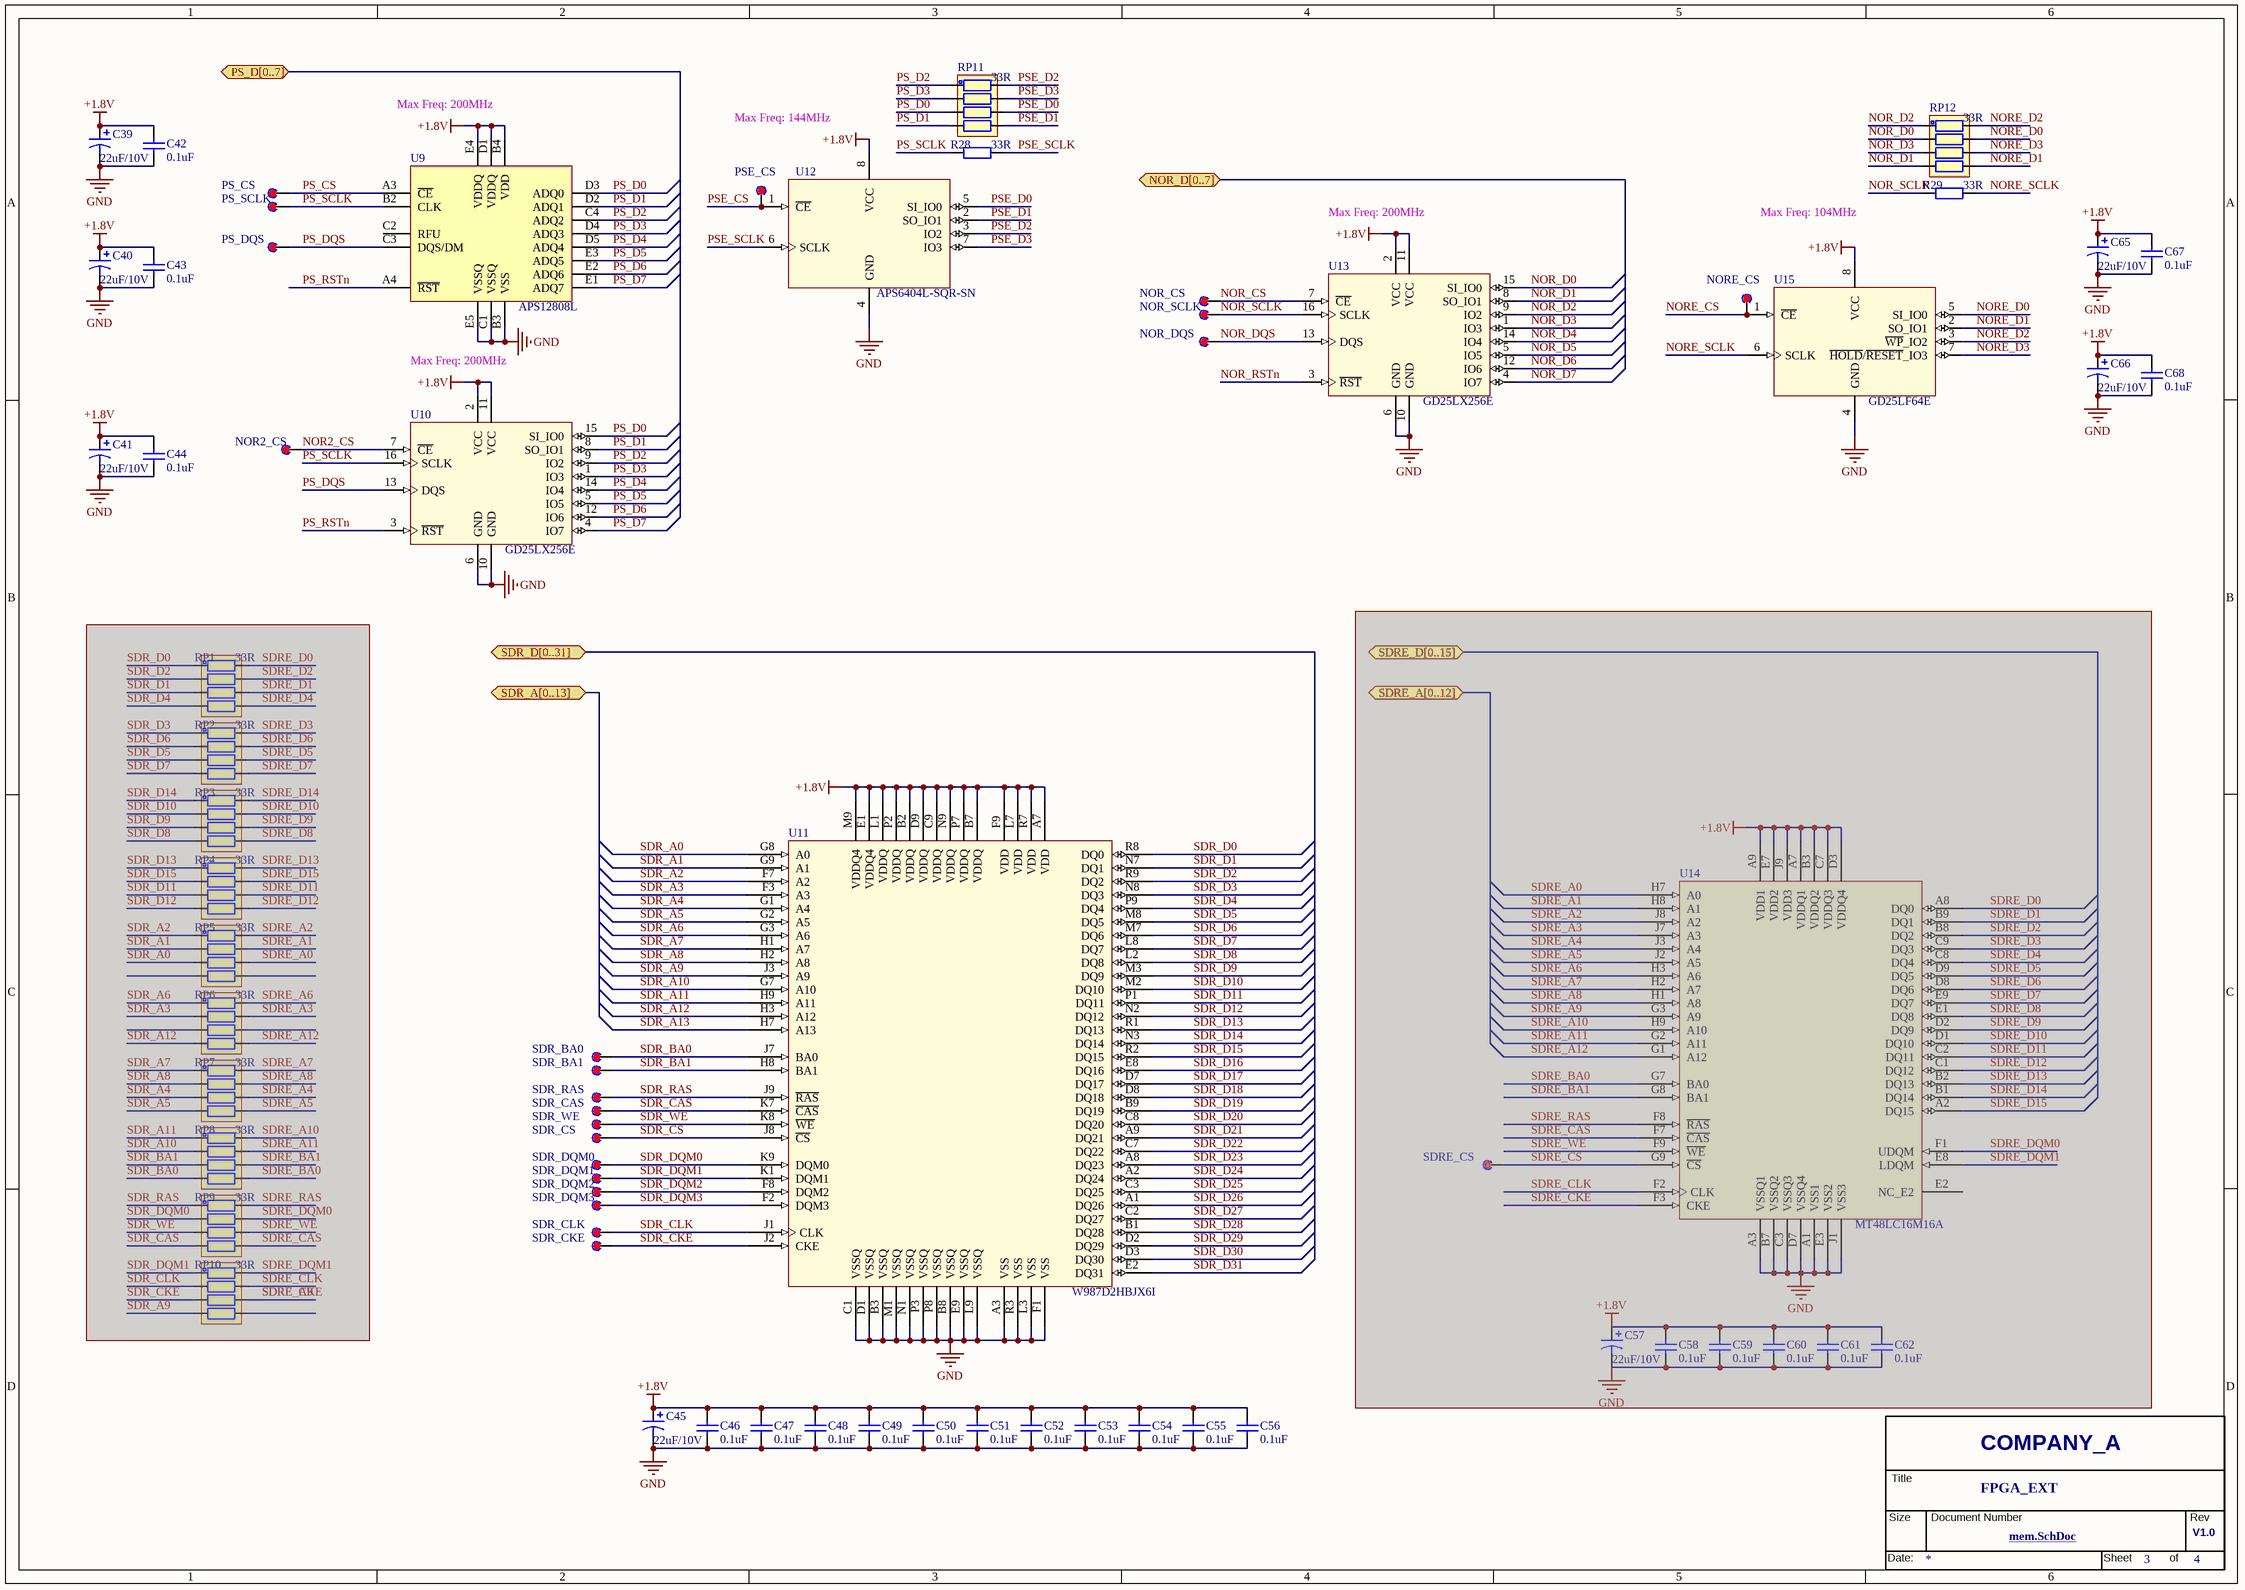
[diagram p0: MISC105414-7.SchDoc]
# Altium project MISC105414-4.PrjPcb (part 2 of 3)
## Sheet MISC105414-7.SchDoc
size 420 x 297 mm; DocumentNumber: MISC105414; SheetNumber: 2; SheetTotal: 4

### Parts
(Parts that share a designator on the sheet are numbered #1, #2 ... from top to bottom, then left to right.)
*?#3  Page Count: 4  Page Number: 3  OrgName: COMPANY_A  Title: FPGA_EXT  RevCode: V1.0  Doc: mem.SchDoc  (hidden comment: TitleBlock_YHSCH)  (graphical)
C39  22uF/10V  [0603C_N]
C40  22uF/10V  [0603C_N]
C41  22uF/10V  [0603C_N]
C42  0.1uF  [0603C_N]
C43  0.1uF  [0603C_N]
C44  0.1uF  [0603C_N]
C45  22uF/10V  [0603C_N]
C46  0.1uF  [0603C_N]
C47  0.1uF  [0603C_N]
C48  0.1uF  [0603C_N]
C49  0.1uF  [0603C_N]
C50  0.1uF  [0603C_N]
C51  0.1uF  [0603C_N]
C52  0.1uF  [0603C_N]
C53  0.1uF  [0603C_N]
C54  0.1uF  [0603C_N]
C55  0.1uF  [0603C_N]
C56  0.1uF  [0603C_N]
C57  22uF/10V  [0603C_N]  (masked out: inside a compile mask, not in the netlist)
C58  0.1uF  [0603C_N]  (masked out: inside a compile mask, not in the netlist)
C59  0.1uF  [0603C_N]  (masked out: inside a compile mask, not in the netlist)
C60  0.1uF  [0603C_N]  (masked out: inside a compile mask, not in the netlist)
C61  0.1uF  [0603C_N]  (masked out: inside a compile mask, not in the netlist)
C62  0.1uF  [0603C_N]  (masked out: inside a compile mask, not in the netlist)
C65  22uF/10V  [0603C_N]
C66  22uF/10V  [0603C_N]
C67  0.1uF  [0603C_N]
C68  0.1uF  [0603C_N]
R28  33R  [0603R_N]
R29  33R  [0603R_N]
RP1  33R  [0402RP-4P]  (masked out: inside a compile mask, not in the netlist)
RP2  33R  [0402RP-4P]  (masked out: inside a compile mask, not in the netlist)
RP3  33R  [0402RP-4P]  (masked out: inside a compile mask, not in the netlist)
RP4  33R  [0402RP-4P]  (masked out: inside a compile mask, not in the netlist)
RP5  33R  [0402RP-4P]  (masked out: inside a compile mask, not in the netlist)
RP6  33R  [0402RP-4P]  (masked out: inside a compile mask, not in the netlist)
RP7  33R  [0402RP-4P]  (masked out: inside a compile mask, not in the netlist)
RP8  33R  [0402RP-4P]  (masked out: inside a compile mask, not in the netlist)
RP9  33R  [0402RP-4P]  (masked out: inside a compile mask, not in the netlist)
RP10  33R  [0402RP-4P]  (masked out: inside a compile mask, not in the netlist)
RP11  33R  [0402RP-4P]
RP12  33R  [0402RP-4P]
TP18  PS_CS  [FZ_TP-SMD-Mini]
TP19  PS_SCLK  [FZ_TP-SMD-Mini]
TP20  PS_DQS  [FZ_TP-SMD-Mini]
TP21  NOR2_CS  [FZ_TP-SMD-Mini]
TP22  SDR_BA0  [FZ_TP-SMD-Mini]
TP23  SDR_BA1  [FZ_TP-SMD-Mini]
TP24  SDR_RAS  [FZ_TP-SMD-Mini]
TP25  SDR_CAS  [FZ_TP-SMD-Mini]
TP26  SDR_WE  [FZ_TP-SMD-Mini]
TP27  SDR_CS  [FZ_TP-SMD-Mini]
TP28  SDR_DQM0  [FZ_TP-SMD-Mini]
TP29  SDR_DQM1  [FZ_TP-SMD-Mini]
TP30  SDR_DQM2  [FZ_TP-SMD-Mini]
TP31  SDR_DQM3  [FZ_TP-SMD-Mini]
TP32  SDR_CLK  [FZ_TP-SMD-Mini]
TP33  SDR_CKE  [FZ_TP-SMD-Mini]
TP34  PSE_CS  [FZ_TP-SMD-Mini]
TP35  NOR_CS  [FZ_TP-SMD-Mini]
TP36  NOR_SCLK  [FZ_TP-SMD-Mini]
TP37  NOR_DQS  [FZ_TP-SMD-Mini]
TP38  SDRE_CS  [FZ_TP-SMD-Mini]  (masked out: inside a compile mask, not in the netlist)
TP39  NORE_CS  [FZ_TP-SMD-Mini]
U9  APS12808L  [PBGA24 6X8]
U10  GD25LX256E  [SOIC16]
U11  W987D2HBJX6I  [VFBGA90_8X13]
U12  APS6404L-SQR-SN  [SOP8]
U13  GD25LX256E  [SOIC16]
U14  MT48LC16M16A  [VFBGA54_8X9]  (masked out: inside a compile mask, not in the netlist)
U15  GD25LF64E  [SOIC8]

### Ports
NOR_D[0..7], PS_D[0..7], SDR_A[0..13], SDR_D[0..31], SDRE_A[0..12], SDRE_D[0..15]

### Nets
+1.8V: C39.1 C40.1 C41.1 C42.2 C43.2 C44.2 C45.1 C46.2 C47.2 C48.2 C49.2 C50.2 C51.2 C52.2 C53.2 C54.2 C55.2 C56.2 C65.1 C66.1 C67.2 C68.2 U9.B4(VDD) U9.D1(VDDQ) U9.E4(VDDQ) U10.2(VCC) U10.11(VCC) U11.A7(VDD) U11.B2(VDDQ) U11.B7(VDDQ) U11.C9(VDDQ) U11.D9(VDDQ) U11.E1(VDDQ4) U11.F9(VDD) U11.L1(VDDQ) U11.L7(VDD) U11.M9(VDDQ4) U11.N9(VDDQ) U11.P2(VDDQ) U11.P7(VDDQ) U11.R7(VDD) U12.8(VCC) U13.2(VCC) U13.11(VCC) U15.8(VCC)
GND: C39.2 C40.2 C41.2 C42.1 C43.1 C44.1 C45.2 C46.1 C47.1 C48.1 C49.1 C50.1 C51.1 C52.1 C53.1 C54.1 C55.1 C56.1 C65.2 C66.2 C67.1 C68.1 U9.B3(VSS) U9.C1(VSSQ) U9.E5(VSSQ) U10.6(GND) U10.10(GND) U11.A3(VSS) U11.B3(VSSQ) U11.B8(VSSQ) U11.C1(VSSQ) U11.D1(VSSQ) U11.E9(VSSQ) U11.F1(VSS) U11.L3(VSS) U11.L9(VSSQ) U11.M1(VSSQ) U11.N1(VSSQ) U11.P3(VSSQ) U11.P8(VSSQ) U11.R3(VSS) U12.4(GND) U13.6(GND) U13.10(GND) U15.4(GND)
NOR2_CS: TP21.1 U10.7(~{CE})
NOR_CS: TP35.1 U13.7(~{CE})
NOR_D0: RP12.2 U13.15(SI_IO0)
NOR_D1: RP12.4 U13.8(SO_IO1)
NOR_D2: RP12.1 U13.9(IO2)
NOR_D3: RP12.3 U13.1(IO3)
NOR_D4: U13.14(IO4)
NOR_D5: U13.5(IO5)
NOR_D6: U13.12(IO6)
NOR_D7: U13.4(IO7)
NOR_DQS: TP37.1 U13.13(DQS)
NOR_RSTn: U13.3(~{RST})
NOR_SCLK: R29.2 TP36.1 U13.16(SCLK)
NORE_CS: TP39.1 U15.1(~{CE})
NORE_D0: RP12.7 U15.5(SI_IO0)
NORE_D1: RP12.5 U15.2(SO_IO1)
NORE_D2: RP12.8 U15.3(~{WP}_IO2)
NORE_D3: RP12.6 U15.7(~{HOLD}/~{RESET}_IO3)
NORE_SCLK: R29.1 U15.6(SCLK)
PS_CS: TP18.1 U9.A3(~{CE})
PS_D0: RP11.3 U9.D3(ADQ0) U10.15(SI_IO0)
PS_D1: RP11.4 U9.D2(ADQ1) U10.8(SO_IO1)
PS_D2: RP11.1 U9.C4(ADQ2) U10.9(IO2)
PS_D3: RP11.2 U9.D4(ADQ3) U10.1(IO3)
PS_D4: U9.D5(ADQ4) U10.14(IO4)
PS_D5: U9.E3(ADQ5) U10.5(IO5)
PS_D6: U9.E2(ADQ6) U10.12(IO6)
PS_D7: U9.E1(ADQ7) U10.4(IO7)
PS_DQS: TP20.1 U9.C3(DQS/DM) U10.13(DQS)
PS_RSTn: U9.A4(~{RST}) U10.3(~{RST})
PS_SCLK: R28.2 TP19.1 U9.B2(CLK) U10.16(SCLK)
PSE_CS: TP34.1 U12.1(~{CE})
PSE_D0: RP11.6 U12.5(SI_IO0)
PSE_D1: RP11.5 U12.2(SO_IO1)
PSE_D2: RP11.8 U12.3(IO2)
PSE_D3: RP11.7 U12.7(IO3)
PSE_SCLK: R28.1 U12.6(SCLK)
SDR_A0: U11.G8(A0)
SDR_A1: U11.G9(A1)
SDR_A2: U11.F7(A2)
SDR_A3: U11.F3(A3)
SDR_A4: U11.G1(A4)
SDR_A5: U11.G2(A5)
SDR_A6: U11.G3(A6)
SDR_A7: U11.H1(A7)
SDR_A8: U11.H2(A8)
SDR_A9: U11.J3(A9)
SDR_A10: U11.G7(A10)
SDR_A11: U11.H9(A11)
SDR_A12: U11.H3(A12)
SDR_A13: U11.H7(A13)
SDR_BA0: TP22.1 U11.J7(BA0)
SDR_BA1: TP23.1 U11.H8(BA1)
SDR_CAS: TP25.1 U11.K7(~{CAS})
SDR_CKE: TP33.1 U11.J2(CKE)
SDR_CLK: TP32.1 U11.J1(CLK)
SDR_CS: TP27.1 U11.J8(~{CS})
SDR_D0: U11.R8(DQ0)
SDR_D1: U11.N7(DQ1)
SDR_D2: U11.R9(DQ2)
SDR_D3: U11.N8(DQ3)
SDR_D4: U11.P9(DQ4)
SDR_D5: U11.M8(DQ5)
SDR_D6: U11.M7(DQ6)
SDR_D7: U11.L8(DQ7)
SDR_D8: U11.L2(DQ8)
SDR_D9: U11.M3(DQ9)
SDR_D10: U11.M2(DQ10)
SDR_D11: U11.P1(DQ11)
SDR_D12: U11.N2(DQ12)
SDR_D13: U11.R1(DQ13)
SDR_D14: U11.N3(DQ14)
SDR_D15: U11.R2(DQ15)
SDR_D16: U11.E8(DQ16)
SDR_D17: U11.D7(DQ17)
SDR_D18: U11.D8(DQ18)
SDR_D19: U11.B9(DQ19)
SDR_D20: U11.C8(DQ20)
SDR_D21: U11.A9(DQ21)
SDR_D22: U11.C7(DQ22)
SDR_D23: U11.A8(DQ23)
SDR_D24: U11.A2(DQ24)
SDR_D25: U11.C3(DQ25)
SDR_D26: U11.A1(DQ26)
SDR_D27: U11.C2(DQ27)
SDR_D28: U11.B1(DQ28)
SDR_D29: U11.D2(DQ29)
SDR_D30: U11.D3(DQ30)
SDR_D31: U11.E2(DQ31)
SDR_DQM0: TP28.1 U11.K9(DQM0)
SDR_DQM1: TP29.1 U11.K1(DQM1)
SDR_DQM2: TP30.1 U11.F8(DQM2)
SDR_DQM3: TP31.1 U11.F2(DQM3)
SDR_RAS: TP24.1 U11.J9(~{RAS})
SDR_WE: TP26.1 U11.K8(~{WE})

Not connected (* = marked no-connect by the designer): U9 C2(RFU)

### Notes on the sheet
- Max Freq: 200MHz
- Max Freq: 144MHz
- Max Freq: 104MHz

### Library data of the parts
*?#3 = TitleBlock_YHSCH: Cage Code: 1; Page Modify Date: *
C39-C41 C45 C57 C65 C66 = Cap Pol1: Polarized Capacitor (Radial); Value: 1uF; Published: 8-Jun-2000; LatestRevisionDate: 17-Jul-2002; LatestRevisionNote: Re-released for DXP Platform.; PackageReference: RB7.6-15; Publisher: Altium Limited
C42-C44 C46-C56 C58-C62 C67 C68 = Cap: Capacitor; Value: 100nF; Published: 8-Jun-2000; LatestRevisionDate: 17-Jul-2002; LatestRevisionNote: Re-released for DXP Platform.; PackageReference: RAD-0.3; Publisher: Altium Limited
R28 R29 = Res2: Resistor; Value: 4.7K; Published: 8-Jun-2000; LatestRevisionDate: 17-Jul-2002; LatestRevisionNote: Re-released for DXP Platform.; PackageReference: AXIAL-0.4; Publisher: Altium Limited
RP1-RP12 = R4P
TP18-TP39 = TP_SMD
U9 = APS12808L_PSRAM: PSRAM
U10 U13 = GD25LX256E_8-line SPI Flash: SPI Flash
U11 = W987D2H_SDRAM: SDRAM, 1.8V, 32bit
U12 = APS6404L_PSRAM
U14 = MT48LC16M16A_SDRAM: SDRAM; CLASS: IC
U15 = W25Q64_SPI Flash: CLASS: IC